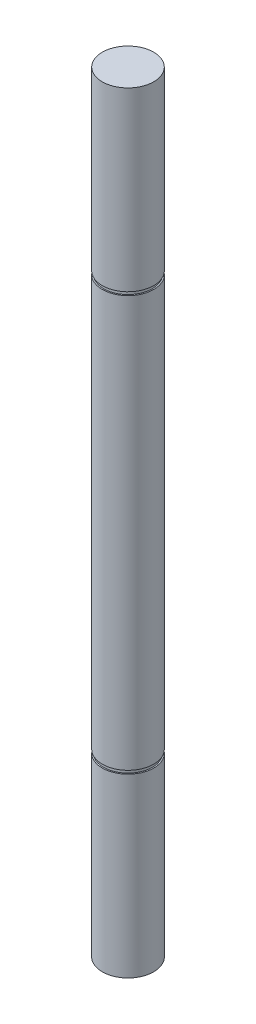
from build123d import *

# Parameters (mm, degrees)
SKETCH_1_R          = 10
EXTRUDE_1_DEPTH     = 300
CUT_EXTRUDE_START   = 1.3
SKETCH_7_R          = 10
SKETCH_7_R_2        = 9.5
CUT_EXTRUDE_3_DEPTH = 1.3
SKETCH_8_R          = 10
SKETCH_8_R_2        = 9.5
CUT_EXTRUDE_4_DEPTH = 1.3
ZJCQC_DEPTH         = 3.5


with BuildPart() as part:
    # 草图1 → 凸台-拉伸1 (new body)
    with BuildSketch(Plane(origin=(0, 0, 0), x_dir=(1, 0, 0), z_dir=(0, 1, 0))):
        with Locations(Location((0, 0, 0), (0, 0, 270))):
            Circle(SKETCH_1_R)
    extrude(amount=EXTRUDE_1_DEPTH)

    # 草图7 → 切除-拉伸3 (cut)
    with BuildSketch(Plane(origin=(0, 70, 0), x_dir=(-1, 0, 0), z_dir=(0, -1, 0)).offset(CUT_EXTRUDE_START)):
        with Locations(Location((0, 0, 0), (0, 0, 90))):
            Circle(SKETCH_7_R)
        with Locations(Location((0, 0, 0), (0, 0, 90))):
            Circle(SKETCH_7_R_2, mode=Mode.SUBTRACT)
    extrude(amount=-CUT_EXTRUDE_3_DEPTH, mode=Mode.SUBTRACT)

    # 草图8 → 切除-拉伸4 (cut)
    with BuildSketch(Plane(origin=(0, 230, 0), x_dir=(1, 0, 0), z_dir=(0, 1, 0))):
        with Locations(Location((0, 0, 0), (0, 0, 90))):
            Circle(SKETCH_8_R)
        with Locations(Location((0, 0, 0), (0, 0, 90))):
            Circle(SKETCH_8_R_2, mode=Mode.SUBTRACT)
    extrude(amount=CUT_EXTRUDE_4_DEPTH, mode=Mode.SUBTRACT)

    # MyToolsZJC → ZJCQC (cut)
    with BuildSketch(Plane.YX.offset(10)):
        with BuildLine():
            Line((148, 3), (152, 3))
            ThreePointArc((152, 3), (155, 0), (152, -3))
            Line((152, -3), (148, -3))
            ThreePointArc((148, -3), (145, 0), (148, 3))
        make_face()
    extrude(amount=-ZJCQC_DEPTH, mode=Mode.SUBTRACT)


solid = part.part
